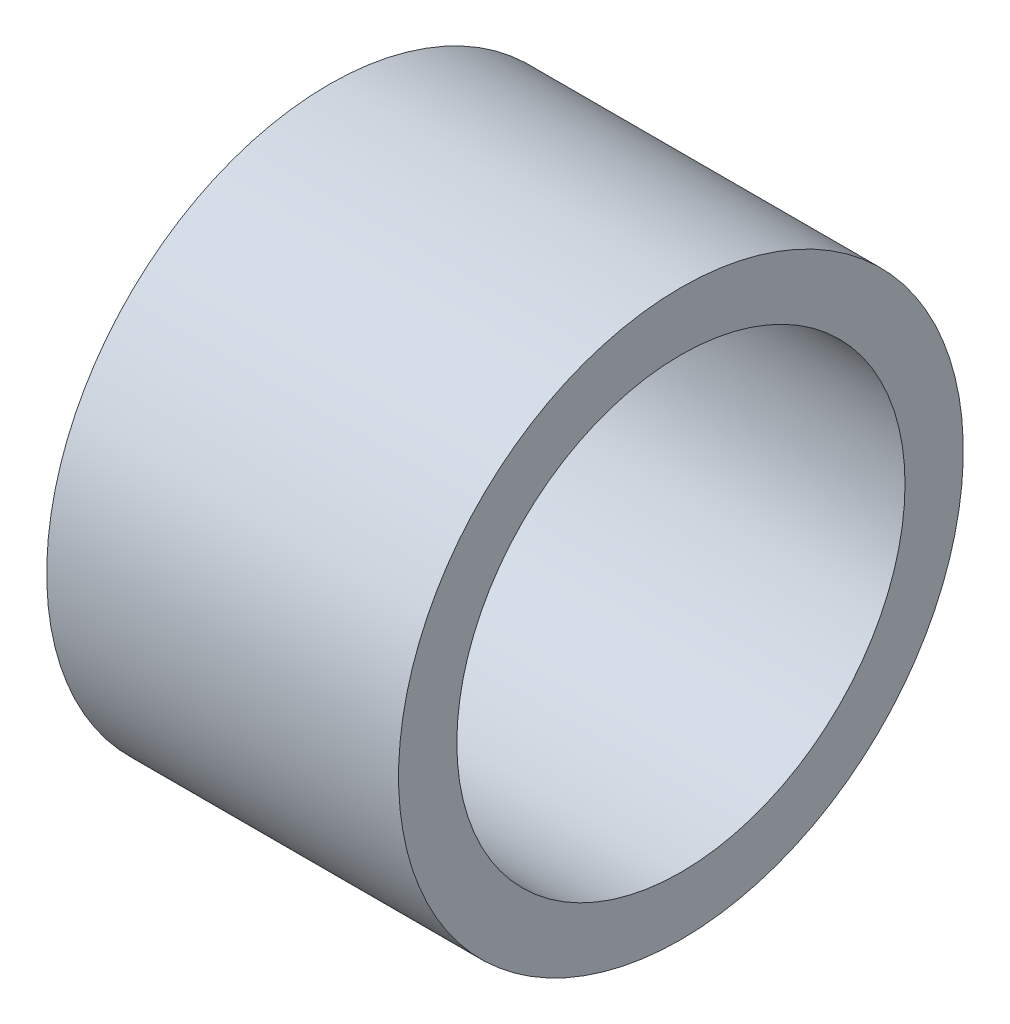
from build123d import *

# Parameters (mm, degrees)
SKETCH1_R           = 31.5
SKETCH1_R_2         = 25
BOSS_EXTRUDE1_DEPTH = 39.25


with BuildPart() as part:
    # Sketch1 → Boss-Extrude1 (new body)
    with BuildSketch(Plane(origin=(191.75, 0, 0), x_dir=(0, 0, -1), z_dir=(1, 0, 0))):
        with Locations(Location((102.5, 90, 0), (0, 0, 90))):
            Circle(SKETCH1_R)
        with Locations(Location((102.5, 90, 0), (0, 0, 90))):
            Circle(SKETCH1_R_2, mode=Mode.SUBTRACT)
    extrude(amount=BOSS_EXTRUDE1_DEPTH)


solid = part.part
